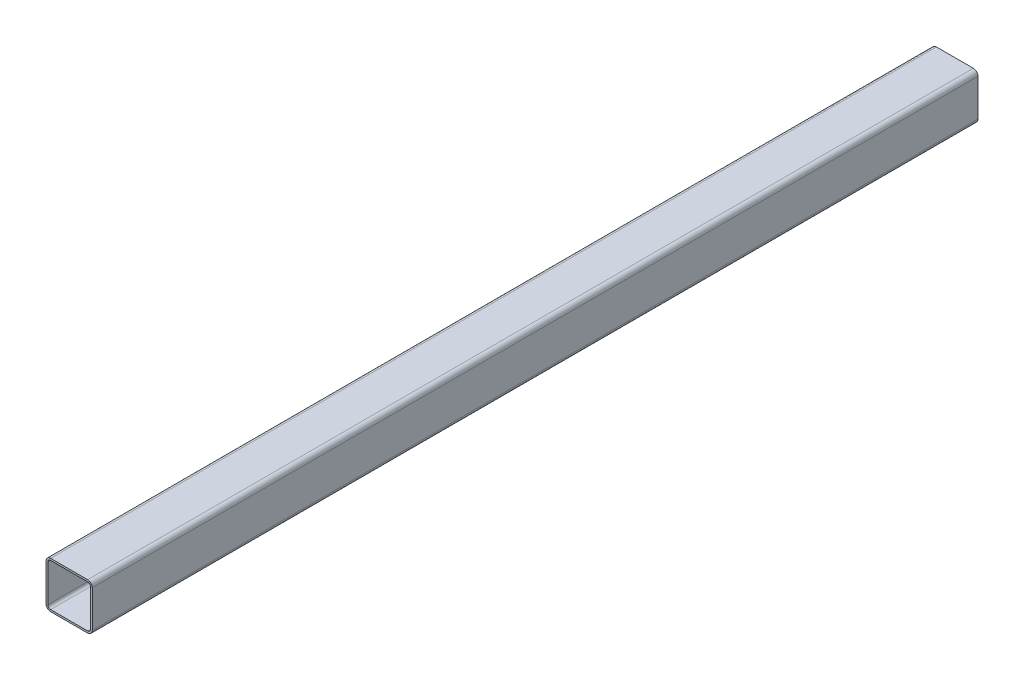
from build123d import *

# Parameters (mm, degrees)
BOSS_EXTRUDE1_DEPTH = 3830


with BuildPart() as part:
    # Sketch1 → Boss-Extrude1 (new body)
    with BuildSketch(Plane.XY):
        with BuildLine():
            Line((-80, 100), (80, 100))
            ThreePointArc((80, 100), (94.142135624, 94.142135624), (100, 80))
            Line((100, 80), (100, -80))
            ThreePointArc((100, -80), (94.142135624, -94.142135624), (80, -100))
            Line((80, -100), (-80, -100))
            ThreePointArc((-80, -100), (-94.142135624, -94.142135624), (-100, -80))
            Line((-100, -80), (-100, 80))
            ThreePointArc((-100, 80), (-94.142135624, 94.142135624), (-80, 100))
        make_face()
        with BuildLine():
            Line((-92, 80), (-92, -80))
            ThreePointArc((-92, -80), (-88.485281374, -88.485281374), (-80, -92))
            Line((-80, -92), (80, -92))
            ThreePointArc((80, -92), (88.485281374, -88.485281374), (92, -80))
            Line((92, -80), (92, 80))
            ThreePointArc((92, 80), (88.485281374, 88.485281374), (80, 92))
            Line((80, 92), (-80, 92))
            ThreePointArc((-80, 92), (-88.485281374, 88.485281374), (-92, 80))
        make_face(mode=Mode.SUBTRACT)
    extrude(amount=BOSS_EXTRUDE1_DEPTH)


solid = part.part
